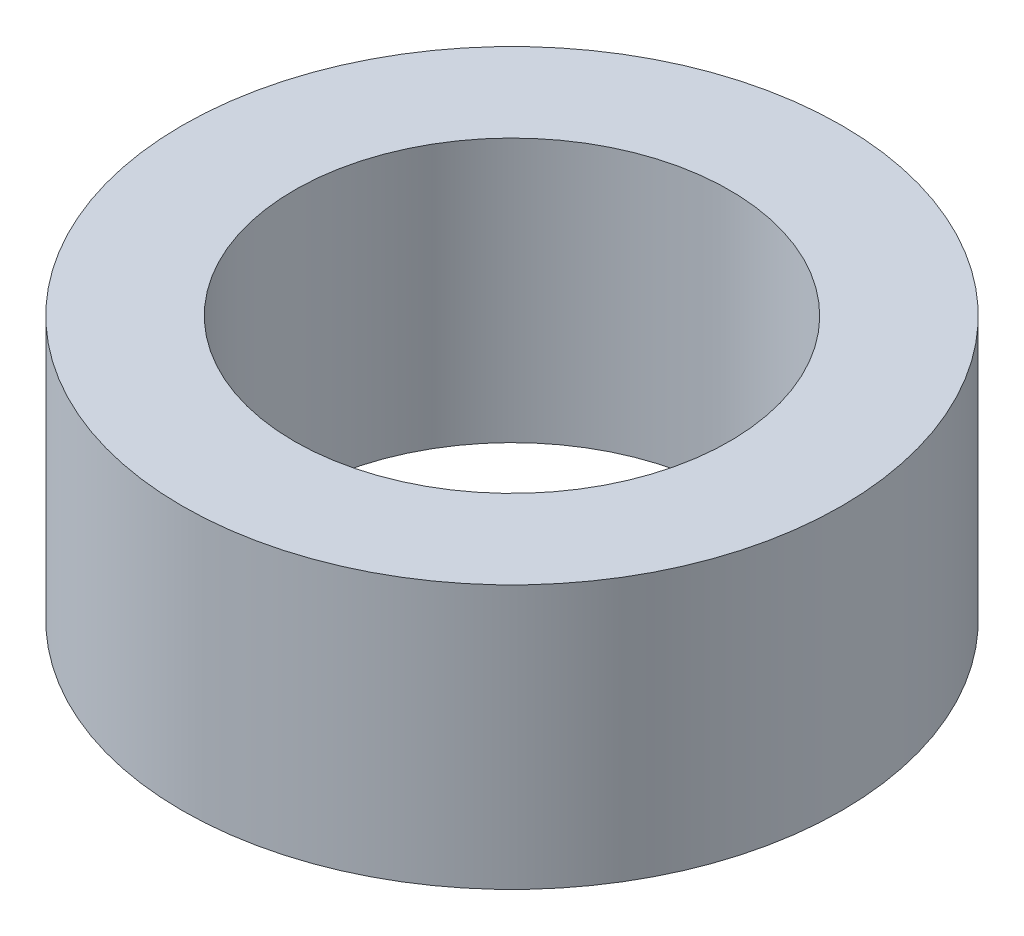
SolidWorks part; units mm, degrees
ref_plane "Front Plane" through (0, 0, 0) normal (0, 0, 1) x (1, 0, 0)
ref_plane "Top Plane" through (0, 0, 0) normal (0, 1, 0) x (1, 0, 0)
ref_plane "Right Plane" through (0, 0, 0) normal (1, 0, 0) x (0, 0, -1)
sketch "Sketch1" plane through (0, 0, 0) normal (0, 1, 0) x (1, 0, 0)
  circle A0 centre (0, 0) radius 8.25
  circle A1 centre (0, 0) radius 12.5
  dimension "D1" = 16.5
  dimension "D2" = 25
extrude "Boss-Extrude1" add sketch "Sketch1" along normal blind 10
